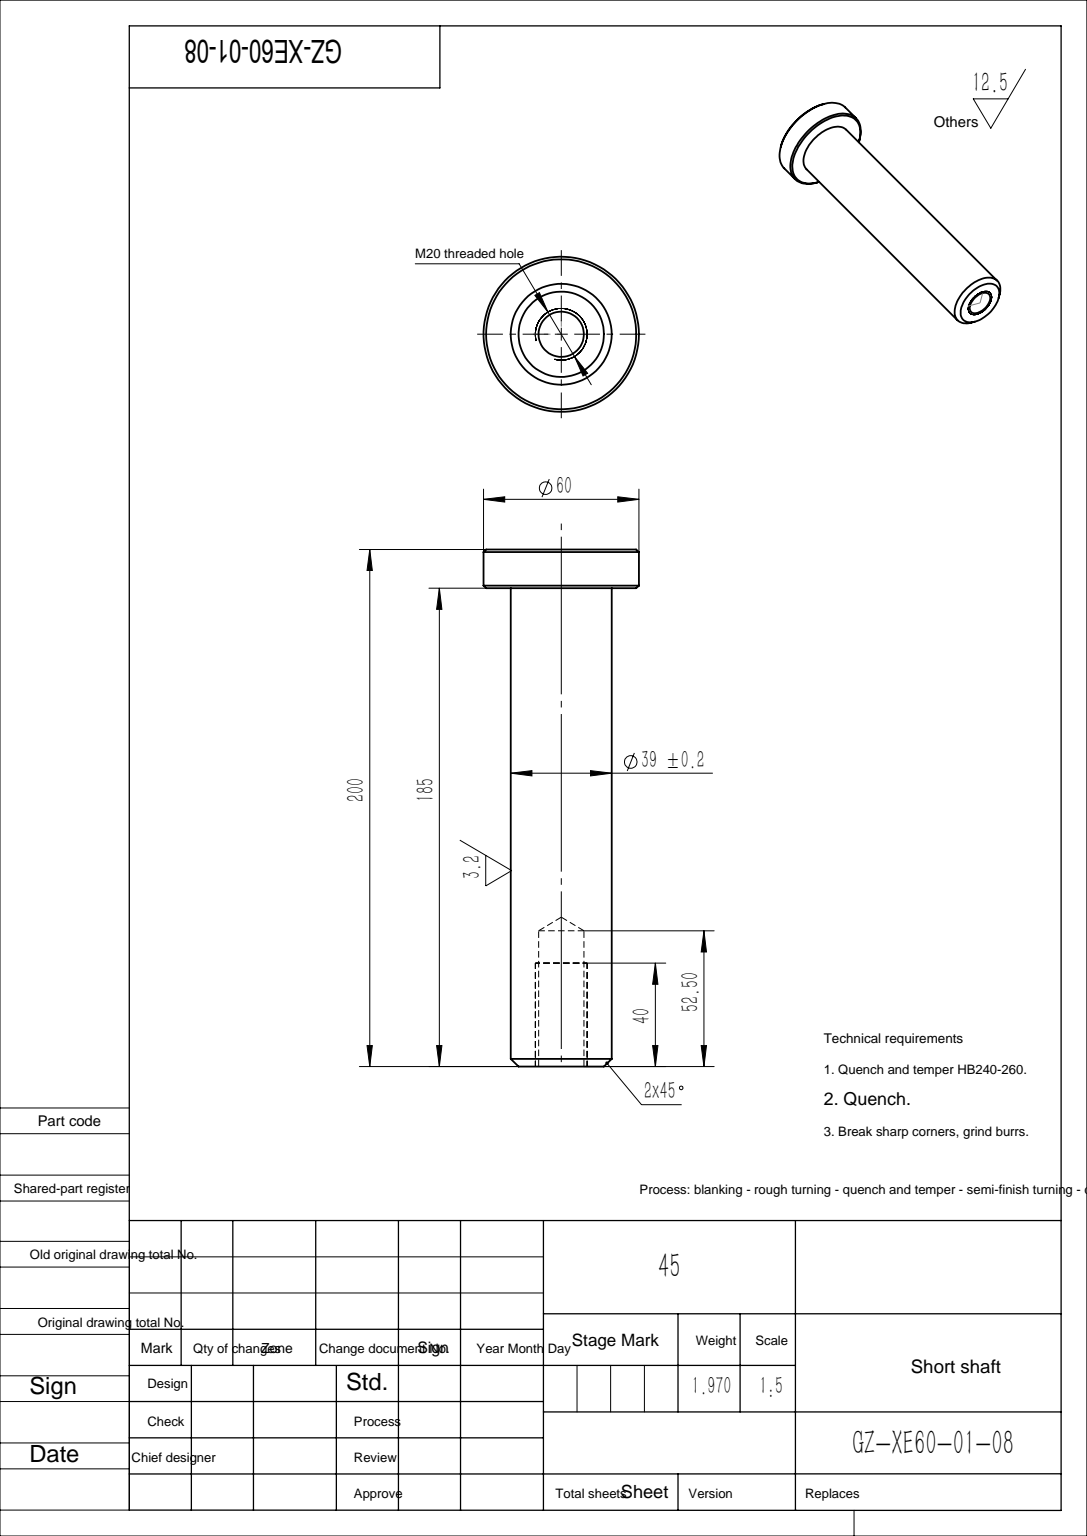
SolidWorks part; units mm, degrees
material "45"
ref_plane "Front Plane" through (0, 0, 0) normal (0, 0, 1) x (1, 0, 0)
ref_plane "Top Plane" through (0, 0, 0) normal (0, 1, 0) x (1, 0, 0)
ref_plane "Right Plane" through (0, 0, 0) normal (1, 0, 0) x (0, 0, -1)
sketch "Sketch1" plane through (0, 0, 0) normal (0, 0, 1) x (1, 0, 0)
  circle A0 centre (0, 0) radius 19.5
  dimension "D1" = 39
extrude "Boss-Extrude1" add sketch "Sketch1" along normal blind 185
sketch "Sketch2" plane through (0, 0, 185) normal (0, 0, 1) x (1, 0, 0)
  circle A0 centre (0, 0) radius 30
  dimension "D1" = 60
extrude "Boss-Extrude2" add sketch "Sketch2" along normal blind 15
chamfer "Chamfer1" distance 3 angle 45 1 edges at (19.5, 0, 0)
chamfer "Chamfer2" distance 1 angle 45 2 edges at (30, 0, 185) (30, 0, 200)
sketch "Sketch3" plane through (0, 0, 0) normal (0, 0, -1) x (-1, 0, 0)
  line L0 (0, 0) -> (10.8876, 0) construction
  line L1 (0, 0) -> (0, -8.3229) construction
hole_wizard "M20 Tapped Hole1" positions "3DSketch1" profile "Sketch4" tap size "M20" standard "GB"
sketch3d "3DSketch1"
  point P0 (0, 0, 0)
  point P3 (0, 0, 0)
  point P5 (0, 0, 0)
  point P7 (0, 0, 0)
sketch "Sketch4" plane through (0, 0, 0) normal (1, 0, 0) x (0, 1, 0)
  line L0 (0, 0) -> (0, 57.7575)
  line L1 (0, 57.7575) -> (8.75, 52.5)
  line L2 (8.75, 52.5) -> (8.75, 0)
  line L5 (8.75, 0) -> (0, 0)
  line L10 (0, 57.7575) -> (-8.75, 52.5) construction
  line L11 (0, -6.35) -> (0, 107.95) construction
  dimension "螺纹孔钻头直径" = 17.5
  dimension "螺纹孔钻头深度" = 52.5
  dimension "导头角度" = 118
cosmetic thread "Cosmetic Thread1" parameters "D1"=40, "D2"=20
cosmetic thread "Cosmetic Thread2" parameters "D1"=40, "D2"=20
cosmetic thread "Cosmetic Thread3" parameters "D1"=40, "D2"=20
cosmetic thread "Cosmetic Thread4" parameters "D1"=40, "D2"=20
